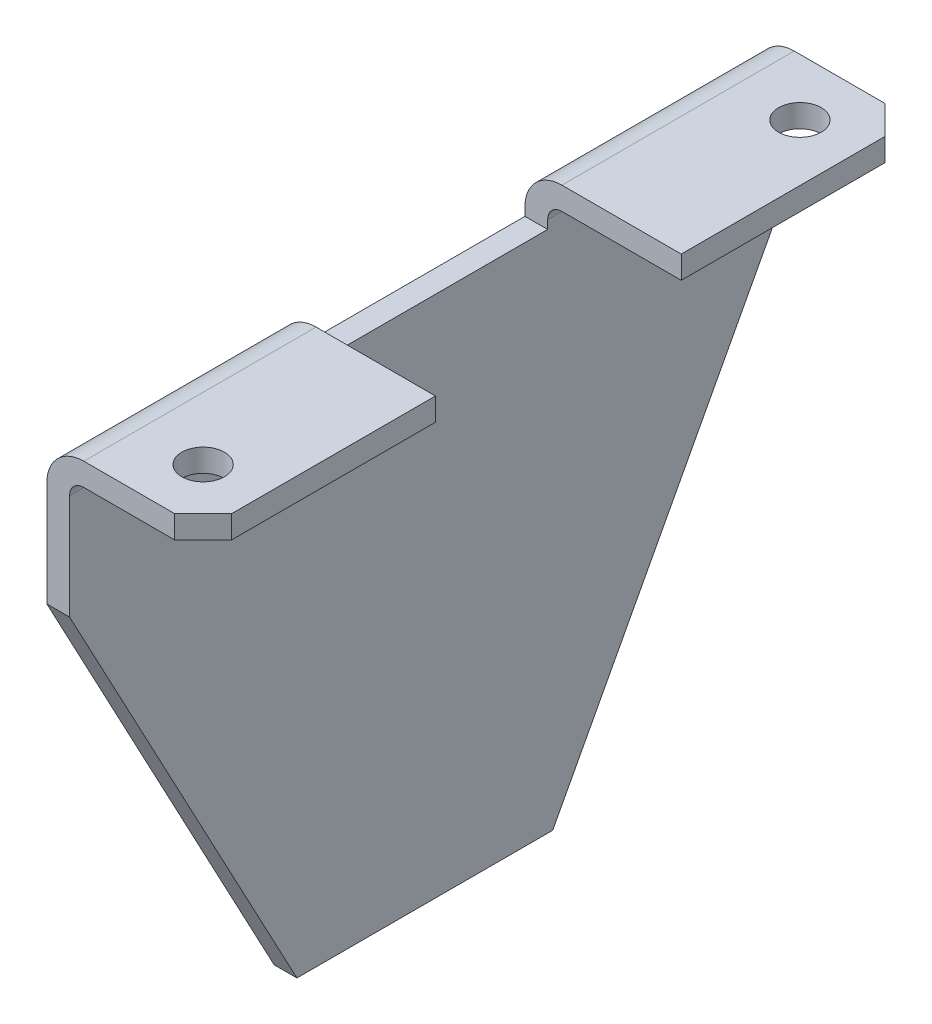
SolidWorks part; units mm, degrees
material "1023 碳钢板 (SS)"
ref_plane "Front Plane" through (0, 0, 0) normal (0, 0, 1) x (1, 0, 0)
ref_plane "Top Plane" through (0, 0, 0) normal (0, 1, 0) x (1, 0, 0)
ref_plane "Right Plane" through (0, 0, 0) normal (1, 0, 0) x (0, 0, -1)
sketch "Sketch1" plane through (0, 0, 0) normal (0, 0, 1) x (1, 0, 0)
  line L0 (0, 0) -> (-42, 0)
  line L5 (-55, -13) -> (-55, -200)
  line L6 (0, -8) -> (-42, -8)
  line L7 (-47, -13) -> (-47, -200)
  line L8 (0, 0) -> (0, -8)
  line L9 (-47, -200) -> (-55, -200)
  arc A0 (-42, 0) -> (-55, -13) centre (-42, -13) ccw
  arc A1 (-42, -8) -> (-47, -13) centre (-42, -13) ccw
  point P6 (-55, 0)
  dimension "D3" = 13
  dimension "D1" = 55
  dimension "D2" = 200
  dimension "D4" = 8
extrude "Boss-Extrude1" add sketch "Sketch1" along normal blind 250 contours L9 L5 A0 L0 L8 L6 A1 L7
sketch "Sketch2" plane through (-55, 0, 0) normal (-1, 0, 0) x (0, 0, 1)
  line L0 (0, -50) -> (80, -200)
  line L1 (0, -13) -> (0, -200) construction
  line L2 (250, -200) -> (0, -200) construction
  line L3 (80, -200) -> (0, -200)
  line L4 (0, -200) -> (0, -50)
  line L5 (125, -200) -> (125, -98.8892) construction
  line L6 (170, -200) -> (250, -200)
  line L7 (250, -50) -> (170, -200)
  line L8 (250, -200) -> (250, -50)
  line L9 (250, 0) -> (0, 0) construction
  line L10 (168.25, -16) -> (81.75, -16)
  line L11 (168.25, -16) -> (168.25, 72.4926)
  line L12 (168.25, 72.4926) -> (81.75, 72.4926)
  line L13 (81.75, -16) -> (81.75, 72.4926)
  line L14 (168.25, -16) -> (81.75, 72.4926) construction
  line L15 (168.25, 72.4926) -> (81.75, -16) construction
  point P12 (125, 28.2463)
  dimension "D1" = 150
  dimension "D2" = 80
  dimension "D3" = 86.5
  dimension "D4" = 16
extrude "Cut-Extrude1" cut sketch "Sketch2" against normal blind 250
sketch "Sketch3" plane through (0, 0, 0) normal (0, 1, 0) x (1, 0, 0)
  line L0 (-55, -81.75) -> (-55, 0) construction
  line L1 (-55, -81.75) -> (-55, -168.25) construction
  line L2 (-55, -125) -> (0, -125) construction
  line L3 (0, 0) -> (-42, 0) construction
  circle A0 centre (-20, -20) radius 7.5
  circle A1 centre (-20, -230) radius 7.5
  dimension "D2" = 15
  dimension "D3" = 210
  dimension "D4" = 105
  dimension "D1" = 35
extrude "Cut-Extrude2" cut sketch "Sketch3" against normal blind 250
chamfer "Chamfer1" distance 10 angle 45 2 edges at (0, -4, 0) (0, -4, 250)
